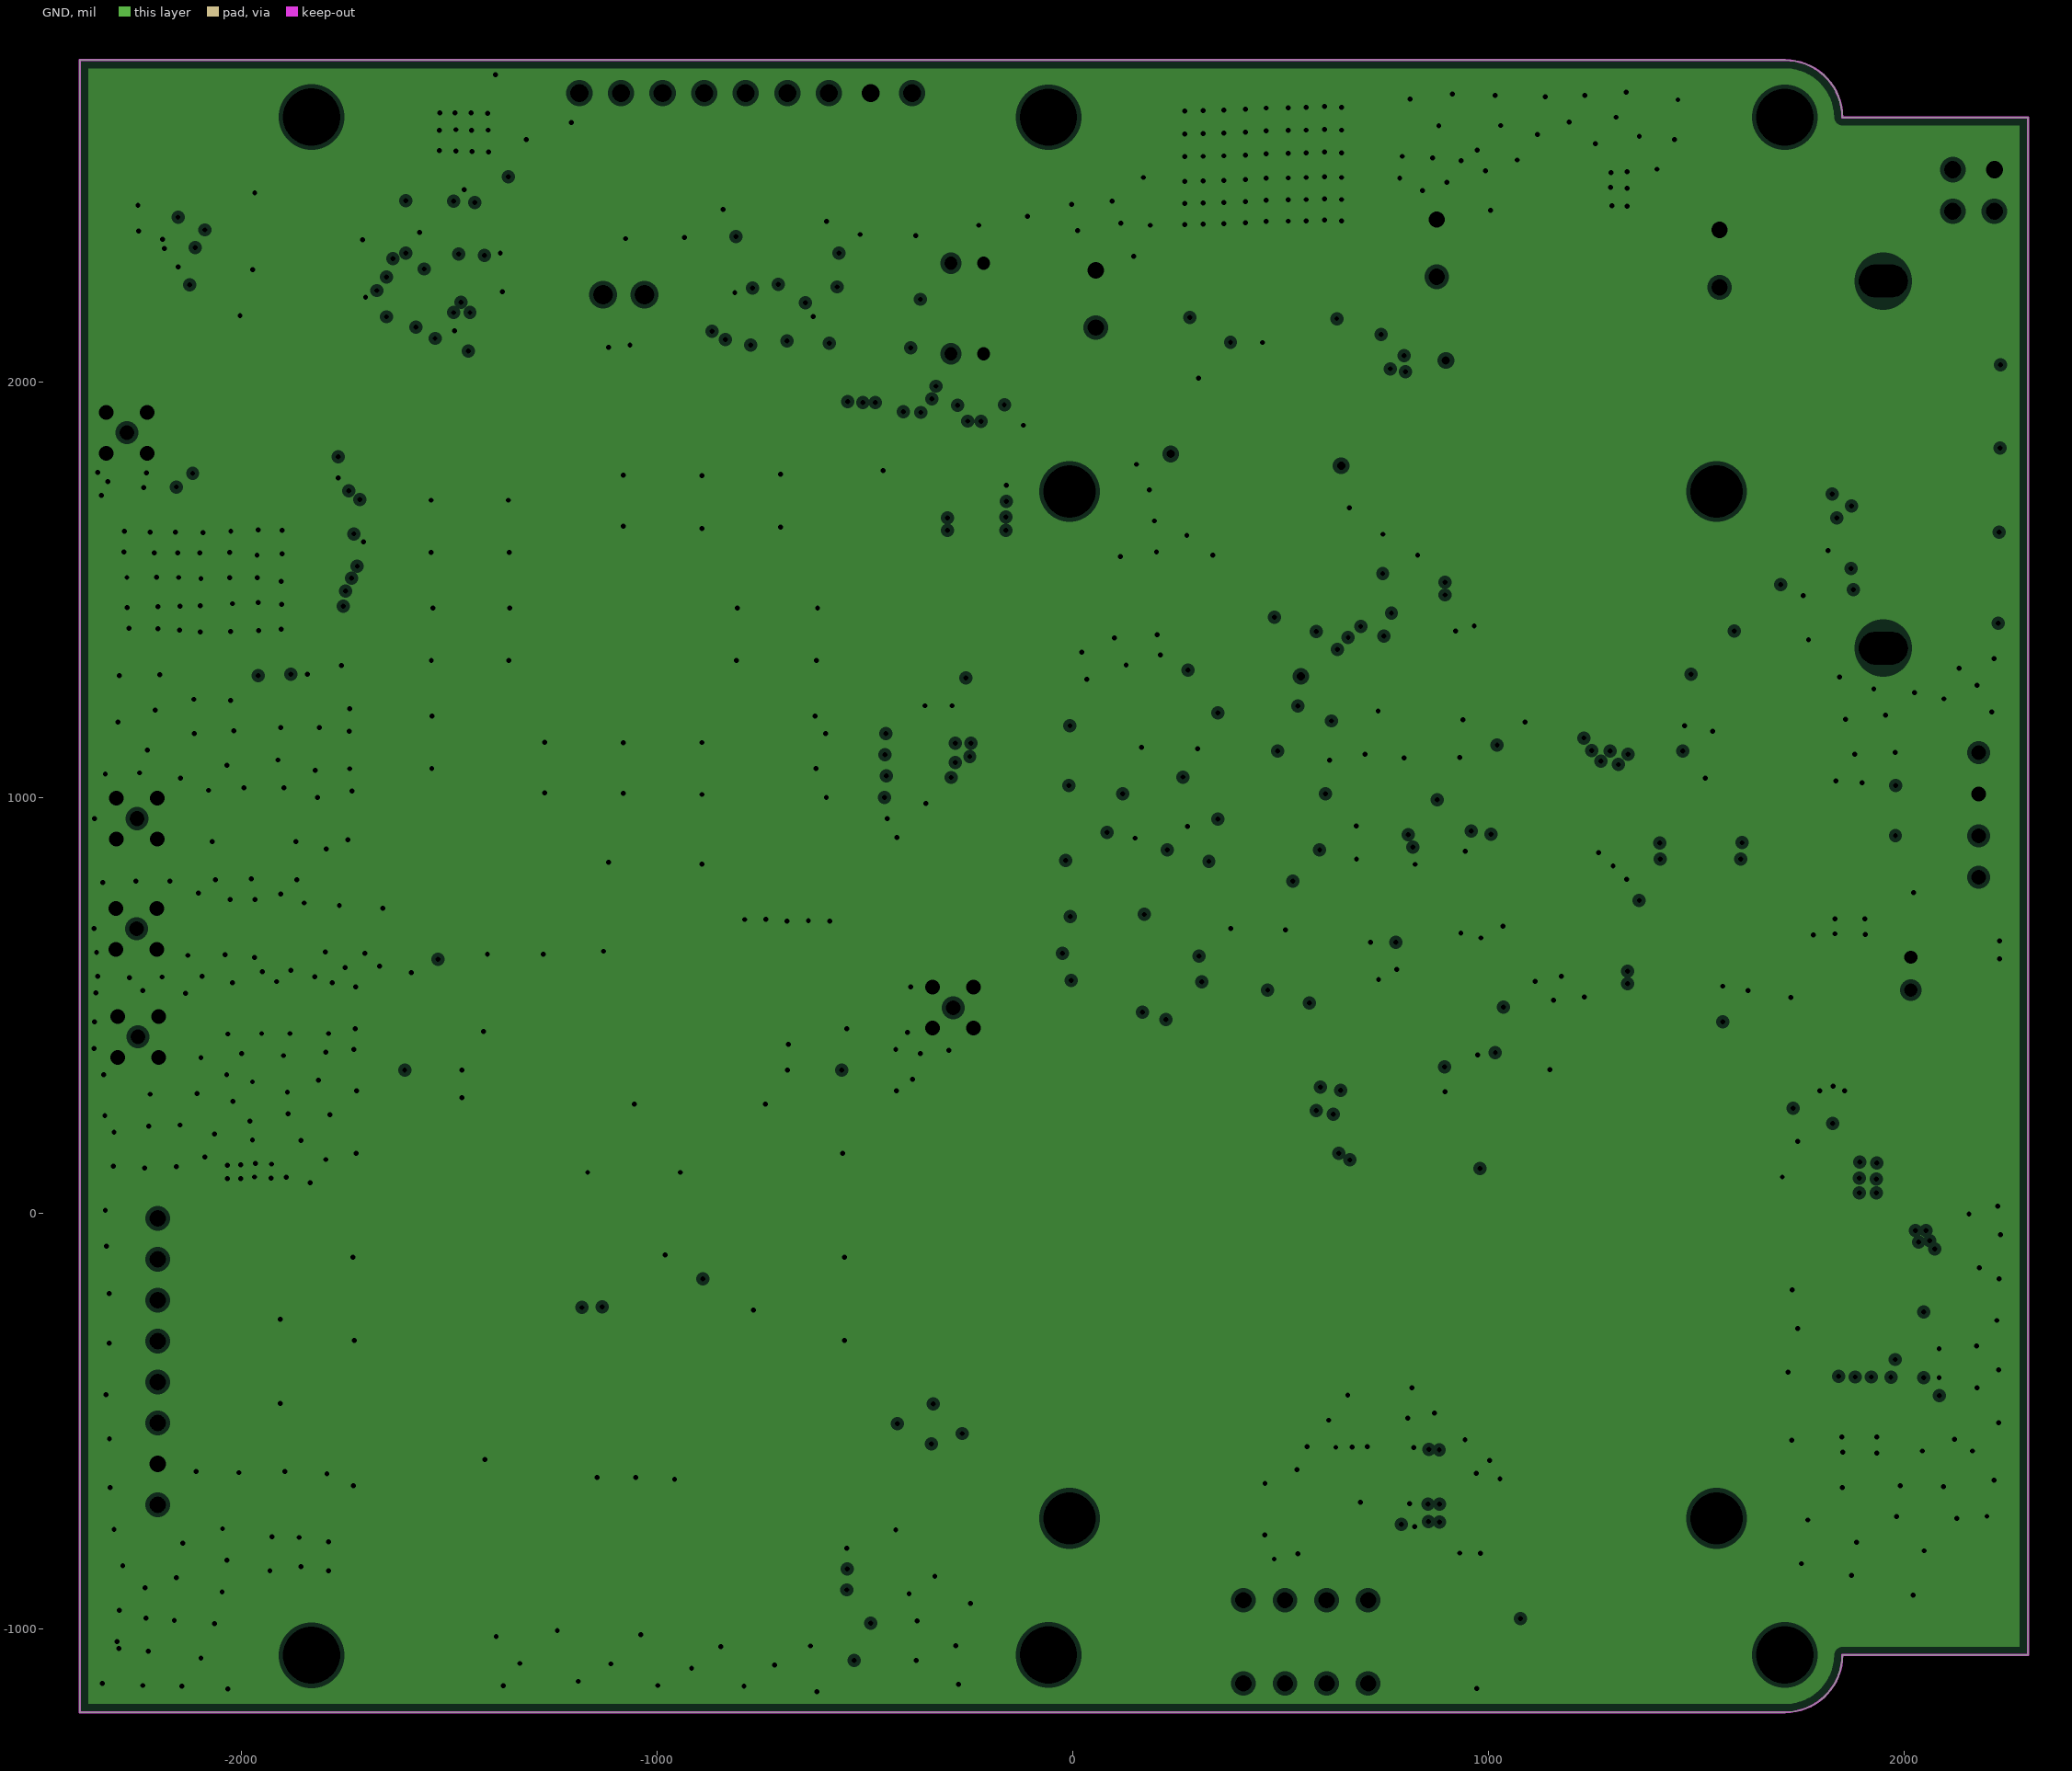
[diagram p0: GND, clearances drawn from the general rule]
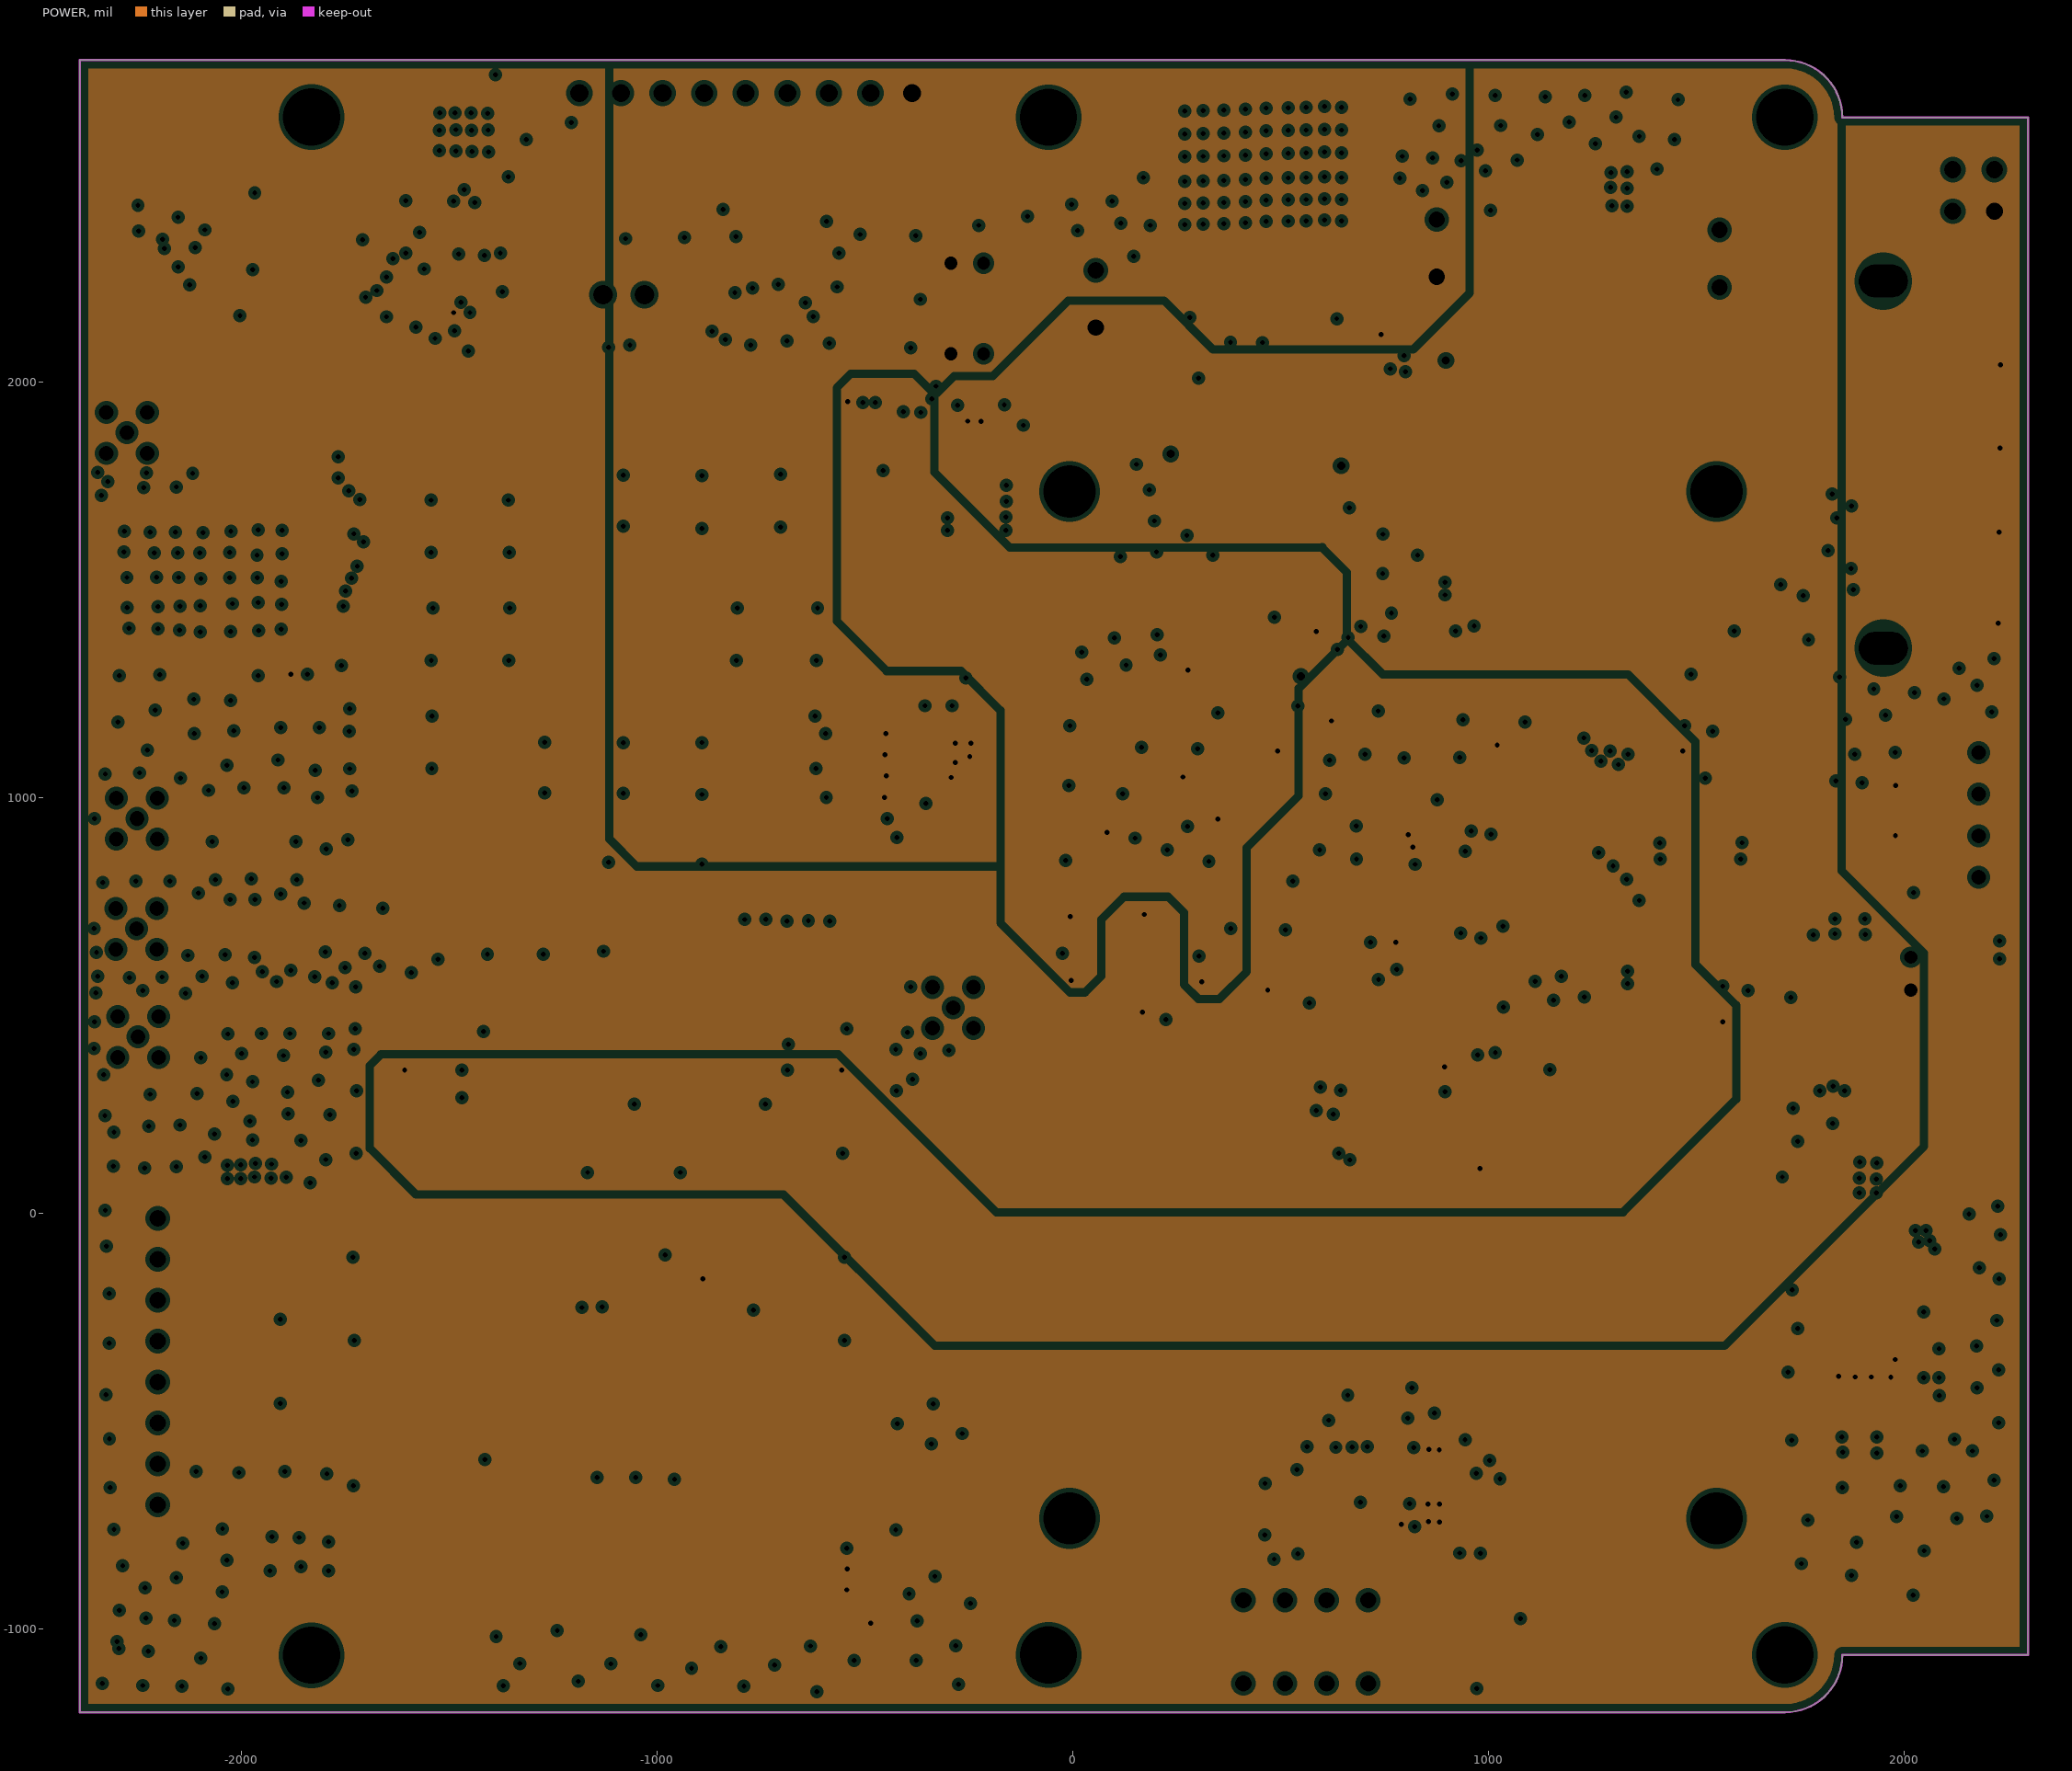
[diagram p1: POWER, clearances drawn from the general rule]
# Altium PCB MISC84456.PcbDoc (part 2 of 5)
## Footprints (in the part's own frame and the unit in brackets; to place one, negate y for a bottom-side part, rotate by r counter-clockwise, add the part's x,y. Pads: shape width x height; smd on the part's side, far side on the other; paste and mask are expansions set on the pad) (continued)
"G6K-2P D12" [mm]
  round 1.8 hole 1: 1(-3.81,-2.54) 2(-1.27,-2.54) 3(1.27,-2.54) 4(3.81,-2.54) 5(3.81,2.54) 6(1.27,2.54) 7(-1.27,2.54) 8(-3.81,2.54)
  silkscreen extent -5.2,-3.4 5.2,3.4
HDR1X4 [mm] "Connector; Header; 4 Position"
  rect 1.5x1.5 hole 0.9: 1(0,0)
  round 1.5 hole 0.9: 2(2.54,0) 3(5.08,0) 4(7.62,0)
  silkscreen extent -1.27,-1.27 8.89,1.27
HLK-B40 [mm]
  rect 1x0.7 smd: 1(-4.75,3.85) 2(-4.75,2.85) 3(-4.75,1.85) 4(-4.75,0.85) 5(-4.75,-0.15) 6(-4.75,-1.15) 7(-4.75,-2.15) 8(-4.75,-3.15) 9(-4.75,-4.15) 10(-4.75,-5.15) 18(4.75,-5.15) 19(4.75,-4.15) 20(4.75,-3.15) 21(4.75,-2.15) 22(4.75,-1.15) 23(4.75,-0.15) 24(4.75,0.85) 25(4.75,1.85) 26(4.75,2.85) 27(4.75,3.85) 28(4.75,4.85) 29(4.75,5.85)
  rect 0.7x1 smd: 11(-3,-5.85) 12(-2,-5.85) 13(-1,-5.85) 14(0,-5.85) 15(1,-5.85) 16(2,-5.85) 17(3,-5.85)
  silkscreen extent -5.97,-5.85 4.75,8.15
HX-DU1006D [mm]
  round 6.2 hole 3.2: 0(-19.75,0.23) 0(19.75,0.23) 2(-19.75,-62.51) 2(19.75,-62.51)
  rect 0.3x2.1 smd: 1(3.5,-2.35) 2(3.5,2.35) 3(3,-2.35) 4(3,2.35) 5(2.5,-2.35) 6(2.5,2.35) 7(2,-2.35) 8(2,2.35) 9(1.5,-2.35) 10(1.5,2.35) 11(1,-2.35) 12(1,2.35) 13(0.5,-2.35) 14(0.5,2.35) 15(0,-2.35) 16(0,2.35) 17(-0.5,-2.35) 18(-0.5,2.35) 19(-1,-2.35) 20(-1,2.35) 21(-1.5,-2.35) 22(-1.5,2.35) 23(-2,-2.35) 24(-2,2.35) 25(-2.5,-2.35) 26(-2.5,2.35) 27(-3,-2.35) 28(-3,2.35) 29(-3.5,-2.35) 30(-3.5,2.35)
  rect 1.6x2.1 smd: 31(-5.9,0) 31(5.9,0)
  silkscreen extent -23.36,-66.07 23.25,3.78
LED0805 [mm] "LED0805"
  rect 0.8x1.3 smd: 1(-0.95,0) 2(0.95,0)
  silkscreen extent -1.6,-0.9 1.6,0.9
LQFP-100_14x14x05P [mm]
  oval 0.3x1.6 smd: 1(-6,-7.55) 2(-5.5,-7.55) 3(-5,-7.55) 4(-4.5,-7.55) 5(-4,-7.55) 6(-3.5,-7.55) 7(-3,-7.55) 8(-2.5,-7.55) 9(-2,-7.55) 10(-1.5,-7.55) 11(-1,-7.55) 12(-0.5,-7.55) 13(0,-7.55) 14(0.5,-7.55) 15(1,-7.55) 16(1.5,-7.55) 17(2,-7.55) 18(2.5,-7.55) 19(3,-7.55) 20(3.5,-7.55) 21(4,-7.55) 22(4.5,-7.55) 23(5,-7.55) 24(5.5,-7.55) 25(6,-7.55) 51(6,7.55) 52(5.5,7.55) 53(5,7.55) 54(4.5,7.55) 55(4,7.55) 56(3.5,7.55) 57(3,7.55) 58(2.5,7.55) 59(2,7.55) 60(1.5,7.55) 61(1,7.55) 62(0.5,7.55) 63(0,7.55) 64(-0.5,7.55) 65(-1,7.55) 66(-1.5,7.55) 67(-2,7.55) 68(-2.5,7.55) 69(-3,7.55) 70(-3.5,7.55) 71(-4,7.55) 72(-4.5,7.55) 73(-5,7.55) 74(-5.5,7.55) 75(-6,7.55)
  oval 1.6x0.3 smd: 26(7.55,-6) 27(7.55,-5.5) 28(7.55,-5) 29(7.55,-4.5) 30(7.55,-4) 31(7.55,-3.5) 32(7.55,-3) 33(7.55,-2.5) 34(7.55,-2) 35(7.55,-1.5) 36(7.55,-1) 37(7.55,-0.5) 38(7.55,0) 39(7.55,0.5) 40(7.55,1) 41(7.55,1.5) 42(7.55,2) 43(7.55,2.5) 44(7.55,3) 45(7.55,3.5) 46(7.55,4) 47(7.55,4.5) 48(7.55,5) 49(7.55,5.5) 50(7.55,6) 76(-7.55,6) 77(-7.55,5.5) 78(-7.55,5) 79(-7.55,4.5) 80(-7.55,4) 81(-7.55,3.5) 82(-7.55,3) 83(-7.55,2.5) 84(-7.55,2) 85(-7.55,1.5) 86(-7.55,1) 87(-7.55,0.5) 88(-7.55,0) 89(-7.55,-0.5) 90(-7.55,-1) 91(-7.55,-1.5) 92(-7.55,-2) 93(-7.55,-2.5) 94(-7.55,-3) 95(-7.55,-3.5) 96(-7.55,-4) 97(-7.55,-4.5) 98(-7.55,-5) 99(-7.55,-5.5) 100(-7.55,-6)
  silkscreen extent -7.03,-8 6.25,6.25
MLP-16 [mm]
  rect 0.23x0.66 smd: 1(-0.6,-0.726)
  rect 0.23x0.56 smd: 2(-0.2,-0.776) 3(0.2,-0.776) 4(0.6,-0.776) 9(0.6,0.776) 10(0.2,0.776) 11(-0.2,0.776) 12(-0.6,0.776)
  rect 0.56x0.23 smd: 5(1.179,-0.6) 6(1.179,-0.2) 7(1.179,0.2) 8(1.179,0.6) 13(-1.179,0.6) 14(-1.179,0.2) 15(-1.179,-0.2) 16(-1.179,-0.6)
  silkscreen extent -1.3,-1.33 1.3,0.9
MMCX-KE [mm]
  round 1.4 hole 0.9: 1(0,0) 2(-1.25,1.25) 3(1.25,1.25) 4(1.25,-1.25) 5(-1.25,-1.25)
  silkscreen extent -1.78,-1.78 1.78,1.78
R0603 [mil]
  rect 30x30 smd: 1(-27.5,0) 2(27.5,0)
  silkscreen extent -52,-25 52,25
R1812 [mil]
  rect 55.38x137.76 smd: 1(-72.97,0) 2(72.97,0)
  silkscreen extent -110,-78 110,78
RB5*7 [mm]
  round 1.3 hole 0.8: 1(-1,0) 2(1,0)
  silkscreen extent -3.83,-2.5 2.5,2.5
RB8*11.5 [mm]
  round 1.6 hole 1: 1(-1.75,0) 2(1.75,0)
  silkscreen extent -5.61,-4 4.04,4
RGB [mm]
  rect 0.55x0.4 smd: 1(0.675,0.725) 2(-0.675,0.725) 5(0.675,-0.725) 6(-0.675,-0.725)
  rect 0.7x0.5 smd: 3(0.75,0) 4(-0.75,0)
  silkscreen extent -0.17,-0.76 1.46,0.82
SMA [mm]
  rect 1.8x2 smd: 1(0,2) 2(0,-2)
  silkscreen extent -1.4,-2.3 1.4,2.3
SMC [mm]
  rect 2.158x3.24 smd: 1(-3.686,0) 2(3.686,0)
  silkscreen extent -4.36,-3.1 3.98,3.1
SMD,4x4x2.6mm [mm]
  rect 1.9x3.7 smd: 1(-2,0) 2(2,0)
  silkscreen extent -2,-2.1 2,2.1
SMD_0.85x0.65mm [mm]
  rect 0.25x0.35 smd: 1(-0.225,0.25) 2(0.225,0.25) 3(0.225,-0.25) 4(-0.225,-0.25)
  silkscreen extent -0.69,-0.5 0.45,0.5
SOP16-6.6 [mil]
  oval 77.6x23.7 smd: 1(-107.7,175) 2(-107.7,125) 3(-107.7,75) 4(-107.7,25) 5(-107.7,-25) 6(-107.7,-75) 7(-107.7,-125) 8(-107.7,-175) 9(107.7,-175) 10(107.7,-125) 11(107.7,-75) 12(107.7,-25) 13(107.7,25) 14(107.7,75) 15(107.7,125) 16(107.7,175)
  silkscreen extent -114,-198 60,211
SOT-23 [mm] "SOT-23"
  rect 0.8x1 smd: 1(-0.95,-1.3) 2(0.95,-1.3) 3(0,1.3)
  silkscreen extent -1.5,-0.61 1.5,0.66
SOT-23_L2.9-W1.3-P1.90-LS2.4-BR [mm]
  rect 1x1.4 smd: 1(-0.95,-1.2) 2(0.95,-1.2) 3(0,1.2)
  silkscreen extent -1.5,-0.7 1.5,0.7
SOT-416_L1.6-W0.8-P1.00-LS1.6-BR [mm]
  rect 0.4x0.7 smd: 1(-0.508,-0.473) 2(0.508,-0.473) 3(0,0.727)
  silkscreen extent -0.85,-0.27 0.85,0.53
SOT-416F_L1.6-W0.8-P1.00-LS1.6-TR [mm]
  rect 0.4x0.7 smd: 1(0.5,-0.7) 2(-0.5,-0.7)
  rect 0.5x0.7 smd: 3(0,0.7)
  silkscreen extent -0.8,-1.48 0.8,0.4
SOT-563 [mm]
  rect 0.545x0.28 smd: 1(-0.723,0.5) 2(-0.723,0) 3(-0.723,-0.5) 4(0.723,-0.5) 5(0.723,0) 6(0.723,0.5)
  silkscreen extent -1.65,-0.88 0.68,0.88
TO-263-5 [mil]
  rect 42.1x90 smd: 1(-134,-183.77) 2(-67,-183.77) 3(0,-183.77) 4(67,-183.77) 5(134,-183.77)
  rect 419.68x350 smd: 6(0,183.77)
  silkscreen extent -200,-188 200,-11
TSOT-23-6 [mm]
  rect 0.8x0.532 smd: 1(1.2,-0.95) 2(1.2,0) 3(1.2,0.95) 4(-1.2,0.95) 5(-1.2,0) 6(-1.2,-0.95)
  silkscreen extent -0.88,-1.82 1.44,1.53
UM482/K823 [mm]
  rect 2.01x0.85 smd: 1(-15,18.415) 2(-15,17.145) 3(-15,15.875) 4(-15,14.605) 5(-15,13.335) 6(-15,12.065) 7(-15,10.795) 8(-15,9.525) 9(-15,8.255) 10(-15,6.985) 11(-15,5.715) 12(-15,4.445) 13(-15,3.175) 14(-15,1.905) 15(-15,0.635) 16(-15,-0.635) 17(-15,-1.905) 18(-15,-3.175) 19(-15,-4.445) 20(-15,-5.715) 21(-15,-6.985) 22(-15,-8.255) 23(-15,-9.525) 24(-15,-10.795) 25(-15,-12.065) 26(-15,-13.335) 27(-15,-14.605) 28(-15,-15.875) 29(-15,-17.145) 30(-15,-18.415) 31(15,-18.415) 32(15,-17.145) 33(15,-15.875) 34(15,-14.605) 35(15,-13.335) 36(15,-12.065) 37(15,-10.795) 38(15,-9.525) 39(15,-8.255) 40(15,-6.985) 41(15,-5.715) 42(15,-4.445) 43(15,-3.175) 44(15,-1.905) 45(15,-0.635) 46(15,0.635) 47(15,1.905) 48(15,3.175) 49(15,4.445) 50(15,5.715) 51(15,6.985) 52(15,8.255) 53(15,9.525) 54(15,10.795) 55(15,12.065) 56(15,13.335) 57(15,14.605) 58(15,15.875) 59(15,17.145) 60(15,18.415)
  silkscreen extent -16.81,-20 15,20
VQFN8 [mm]
  rect 0.8x0.6 smd: 1(-2.7,1.905) 2(-2.7,0.635) 3(-2.7,-0.635) 4(-2.7,-1.905) 5(2.7,-1.905) 6(2.7,-0.635) 7(2.7,0.635) 8(2.7,1.905)
  rect 3.3x3.9 smd: 9(0,0)
  silkscreen extent -3.92,-2.5 3,2.63
XH-8A [mm]
  rect 1.6x1.6 hole 1: 1(-8.75,0)
  round 1.6 hole 1: 2(-6.25,0) 3(-3.75,0) 4(-1.25,0) 5(1.25,0) 6(3.75,0) 7(6.25,0) 8(8.75,0)
  silkscreen extent -11.25,-3.46 11.25,2.35

## Part data
C1 C2 C3 C11 C53 C54 C55 C56: library part Cap, "SMD capacitor"
C4 C91 C104: library part Cap, "470μF,25V,Ф8×11.5mm,RoHS"
C5 C10 C22 C30 C44: library part Cap, "SMD ceramic capacitor,X7R"
C6 C7 C8 C9 C20 C21 C23 C24 C25 C27 C31 C32 C33 C34 C35 C36 C37 C38 C39 C41 C45 C46 C47 C48 C49 C50 C51 C52 C57 C58 C59 C60 C61 C62 C63 C64 C70 C71 C72 C73 C74 C75 C97 C98 C101 C102 C103 C105: library part Cap, "SMD ceramic capacitor"
C26 C28 C40 C42 C43: library part Cap, "SMD ceramic capacitor,X5R"
C29 C76 C77: library part Cap2, "100μF,10V,Ф5×7mm,RoHS"
C87 C88 C92 C93 C94 C95 C96 C99 C100: library part Cap, "SMD capacitor,X7R"
D1 D3: library part Diode, "Default Diode"
D2 D11 D12 D13: library part LED1_3, "Full-color RGB LED,19-337C/RSBHGHC-M03/2T"
D7: library part LED1, "Typical RED GaAs LED"
D8 D14 D15 D16 D17 D18 D19 D24: library part Diode_1, "SMD TVS diode"
J1 J2 J4 J19 J21: library part CIRCLE
J3: library part UM482
J5: library part 2.54
K1: library part Relay-DPDT, "G6K-2P D12,OMRON"
L2: library part Inductor, "Ferrite bead"
L3 L4: library part Inductor, "SMD power inductor,cjiang(Changjiang Micro),FNR4026S2R2MT"
P1: "Header, 4-Pin"
P2: library part "Header 8", "Header, 8-Pin"
Q2: library part PNP, "PNP Bipolar Transistor"
R1 R2 R3 R18 R41 R44 R45 R46 R49 R53 R55 R75 R76 R81 R82 R85 R86 R91 R92 R94: library part Res1, "SMD resistor"
R4 R35 R36 R37 R38: library part Res, "SMD resistor"
R7 R11 R12 R13 R14 R15 R16 R17 R19 R20 R21 R22 R23 R24 R25 R26 R27 R28 R29 R30 R31 R32 R33 R34 R39 R40 R42 R43 R47 R48 R50 R51 R52 R54 R56 R57 R62 R64 R65 R66 R67 R68 R77: library part Res1, "Resistor"
R10: library part RES, "Resettable fuse"
R59 R60 R61 R63: library part RES, "SMD resistor"
U1: "BLE5.1 Bluetooth module,Shenzhen Hi-Link"
U2: library part HX-DU1006D, "Kyocera Japan, 5046 series, mates HX-DU1006D"
U8: library part STM32F103VBH6, "Integrated IC"
U12: library part SP202ECT
U13 U14: library part PESD12VL2BT
U17: library part EC25/EC21
U20 U25: library part SIM-A
U24: library part FSA2567

## Free pads (board coordinates)
  round 275.59 hole 137.8: 0(-1830.71,-1062.24) 0(-1830.71,2637.76) 0(-58.71,-1061.24) 0(-58.71,2636.76) 0(1712.29,-1061.24) 0(1712.29,2636.76)
  round 40 hole 78.74 slot 118.11 at 0 deg unplated: 0(1949,1360) 0(1949,2243)
  round 39.37 smd mask+39.37: MARK(-2269,2661) MARK(-1545,-1107) MARK(2190,-956)
  round 39.37 smd far side mask+39.37: MARK(-2269,2661) MARK(-1545,-1107) MARK(2189,-955)

## Via types
v1: diameter 24, hole 12, TOP to BOTTOM, 400 vias
v2: diameter 24, hole 12, TOP to BOTTOM, tented both sides, 388 vias
v3: diameter 40, hole 20, TOP to BOTTOM, 4 vias

## Nets (pads, with @x,y where several pads share a name; then routed paths per layer and width w, separated by ;. In a path a pad name is that pad's centre, name@x,y a point inside that pad or via, vN(x,y) a via of type N, cw(c..) or ccw(c..) an arc to the next point about the centre after c; other vN are vias at no path point)
232RX-DB: P2.6 R63.1 U14.1 | length 969.2
  BOTTOM w6: P2.6@-2191.4,-494.4 U14.1@-2048.18,-494.4 ; U14.1@-2038,-503 -2017,-524 -1719,-524 -1602,-641 -1354,-641 R63.1@-1294,-581